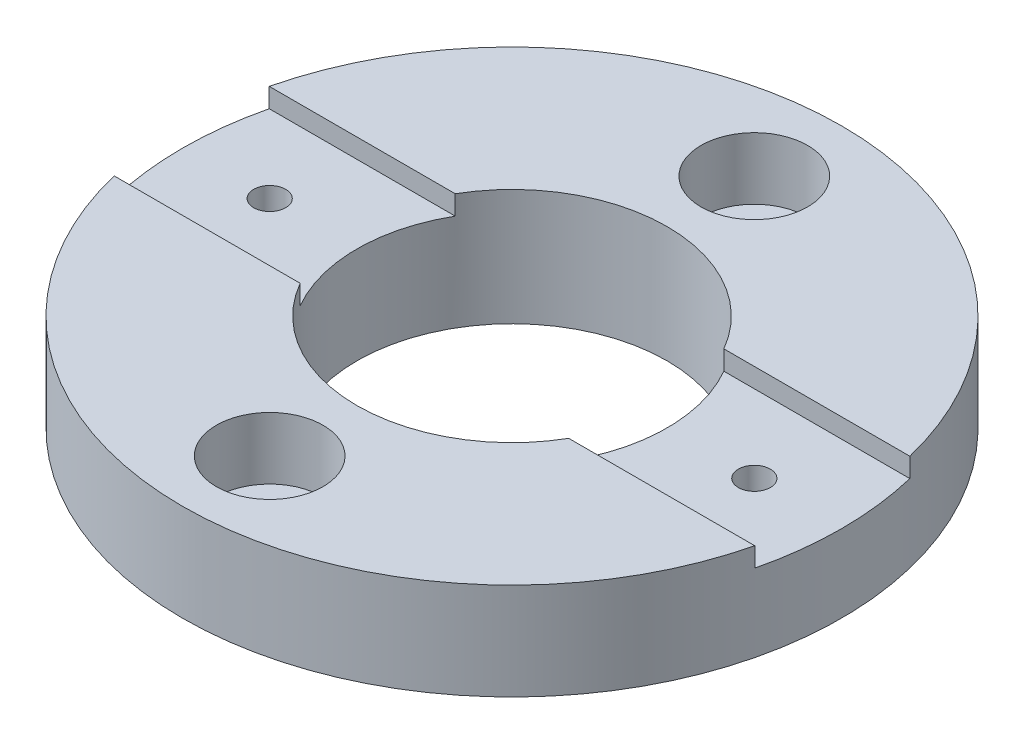
SolidWorks part; units mm, degrees
material "AISI 304"
ref_plane "前视基准面" through (0, 0, 0) normal (0, 0, 1) x (1, 0, 0)
ref_plane "上视基准面" through (0, 0, 0) normal (0, 1, 0) x (1, 0, 0)
ref_plane "右视基准面" through (0, 0, 0) normal (1, 0, 0) x (0, 0, -1)
sketch "草图1" plane through (0, 0, 0) normal (0, 0, 1) x (1, 0, 0)
  line L0 (0, 0) -> (0, 46) construction
  line L1 (0, 46) -> (34, 46)
  line L2 (34, 46) -> (34, 36)
  line L3 (34, 36) -> (18.4, 36)
  line L4 (18.4, 36) -> (18.4, 26)
  line L5 (0, 0) -> (0, 46)
  line L6 (17.4921, 0) -> (0, 0)
  line L7 (18.4, 26) -> (17.4921, 0)
  dimension "D1" = 68
  dimension "D2" = 36.8
  dimension "D3" = 46
  dimension "D4" = 10
  dimension "D5" = 2
  dimension "D6" = 10
revolve "旋转1" add sketch "草图1" angle 360 about L0
sketch "草图2" plane through (0, 46, 0) normal (0, 1, 0) x (1, 0, 0)
  line L0 (0, 25) -> (0, 0) construction
  line L1 (0, 0) -> (0, -25) construction
  point P0 (0, 25)
  point P2 (0, -25)
  dimension "D1" = 50
hole_wizard "M6 六角凹头螺钉的柱形沉头孔1" positions "草图2" profile "草图3" counterbore size "M6" standard "ISO" end condition through all
sketch "草图3" plane through (0, 46, -25) normal (1, 0, 0) x (0, 0, 1)
  line L0 (0, 0) -> (0, 46)
  line L1 (0, 46) -> (3.3, 46)
  line L3 (3.3, 46) -> (3.3, 6.4)
  line L4 (3.3, 6.4) -> (5.5, 6.4)
  line L5 (5.5, 6.4) -> (5.5, 0)
  line L7 (5.5, 0) -> (0, 0)
  line L11 (0, -6.35) -> (0, 107.95) construction
  dimension "通孔孔直径" = 6.6
  dimension "通孔孔深度" = 46
  dimension "柱形沉头孔直径" = 11
  dimension "柱形沉头孔深度" = 6.4
sketch "草图4" plane through (0, 46, 0) normal (0, 1, 0) x (1, 0, 0)
  circle A0 centre (0, 0) radius 16
  dimension "D1" = 32
extrude "切除-拉伸1" cut sketch "草图4" against normal through all
sketch "草图5" plane through (0, 46, 0) normal (0, 1, 0) x (1, 0, 0)
  line L0 (33.0454, -8) -> (13.8564, -8)
  line L1 (0, 0) -> (16, 0) construction
  line L2 (0, 0) -> (0, -34) construction
  line L3 (33.0454, 8) -> (13.8564, 8)
  line L4 (-33.0454, 8) -> (-13.8564, 8)
  line L5 (-33.0454, -8) -> (-13.8564, -8)
  circle A0 centre (0, 0) radius 16 construction
  circle A1 centre (0, 0) radius 34 construction
  arc A2 (13.8564, -8) -> (13.8564, 8) centre (0, 0) ccw
  arc A3 (33.0454, -8) -> (33.0454, 8) centre (0, 0) ccw
  arc A4 (-13.8564, 8) -> (-13.8564, -8) centre (0, 0) ccw
  arc A5 (-33.0454, 8) -> (-33.0454, -8) centre (0, 0) ccw
  point P15 (23.4509, 8)
  dimension "D1" = 16
extrude "凸台-拉伸1" add sketch "草图5" along normal blind 10
sketch "草图6" plane through (0, 56, 0) normal (0, 1, 0) x (1, 0, 0)
  line L0 (13.8564, -8) -> (33.0454, -8) construction
  line L1 (19, -8) -> (-19, -8)
  line L2 (19, -8) -> (19, 8)
  line L3 (19, 8) -> (-19, 8)
  line L4 (-19, -8) -> (-19, 8)
  line L5 (-13.8564, 8) -> (-33.0454, 8) construction
  line L6 (0, 0) -> (0, -8) construction
  dimension "D1" = 38
extrude "切除-拉伸2" cut sketch "草图6" against normal up to surface (10 mm away) up to face at (0, 46, -19.5)
sketch "草图7" plane through (0, 0, 0) normal (1, 0, 0) x (0, 0, -1)
  line L0 (-17.4921, 0) -> (17.4921, 0) construction
  circle A0 centre (0, 50) radius 2
  dimension "D1" = 4
  dimension "D2" = 50
extrude "切除-拉伸3" cut sketch "草图7" against normal through all both and the other way through all
sketch "草图9" plane through (0, 0, 0) normal (0, -1, 0) x (1, 0, 0)
  circle A0 centre (0, 0) radius 20
  dimension "D1" = 40
extrude "切除-拉伸5" cut sketch "草图9" against normal offset from surface (34 mm away) 2 up to face at (0, 36, -28.3)
sketch "草图10" plane through (0, 56, 0) normal (0, 1, 0) x (1, 0, 0)
  line L1 (-50, 8) -> (50, 8)
  line L2 (-50, 8) -> (-50, -8)
  line L3 (-50, -8) -> (50, -8)
  line L4 (50, 8) -> (50, -8)
  line L5 (-50, 8) -> (50, -8) construction
  line L6 (-50, -8) -> (50, 8) construction
  point P0 (0, 0)
  dimension "D1" = 16
  dimension "D2" = 100
extrude "切除-拉伸6" cut sketch "草图10" against normal offset from surface (12 mm away) 2
hole_wizard "M4 螺纹孔1" positions "草图11" profile "草图12" tap size "M4" standard "ISO" end condition through all
sketch "草图11" plane through (0, 46, 0) normal (0, 1, 0) x (1, 0, 0)
  line L0 (-25, 0) -> (0, 0) construction
  line L1 (0, 0) -> (25, 0) construction
  point P0 (-25, 0)
  point P2 (25, 0)
  dimension "D1" = 50
sketch "草图12" plane through (-25, 46, 0) normal (1, 0, 0) x (0, 0, 1)
  line L0 (0, 0) -> (0, 12)
  line L1 (0, 12) -> (1.65, 12)
  line L2 (1.65, 12) -> (1.65, 0)
  line L5 (1.65, 0) -> (0, 0)
  line L11 (0, -6.35) -> (0, 107.95) construction
  dimension "通孔螺纹孔钻头直径" = 3.3
  dimension "通孔螺纹孔钻头深度" = 12
cosmetic thread "孔螺蚊线1" parameters "D2"=4
cosmetic thread "孔螺蚊线2" parameters "D2"=4
